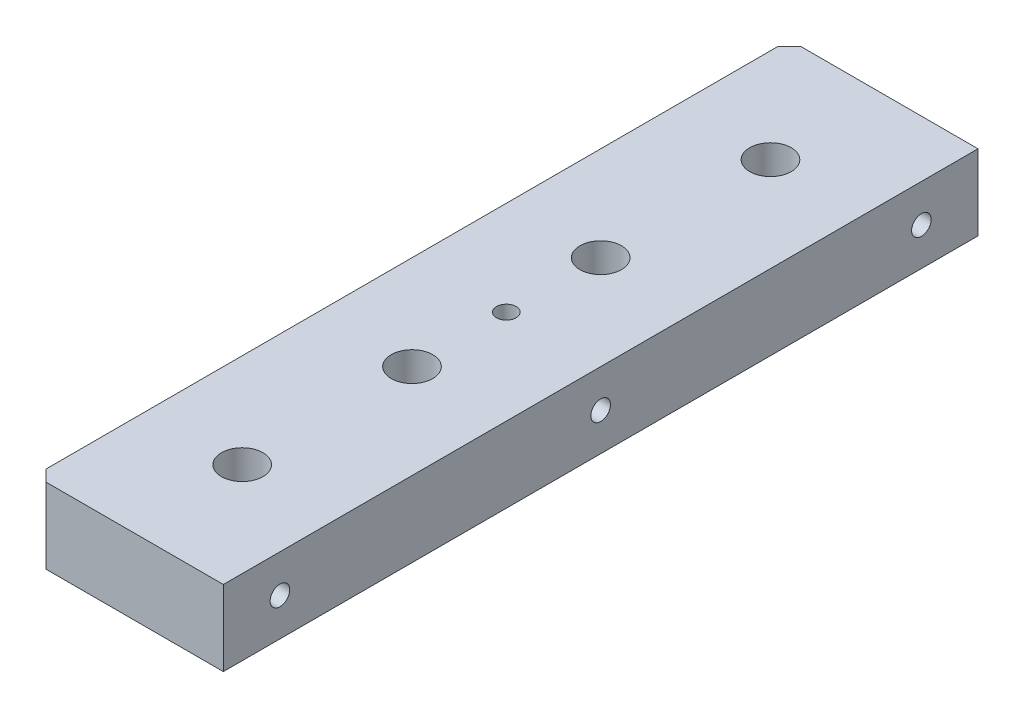
from build123d import *

# Parameters (mm, degrees)
SKETCH_1_W                   = 50
SKETCH_1_H                   = 200
EXTRUDE_1_DEPTH              = 10
HOLE_WIZARD_M6_1_D           = 6.6
HOLE_WIZARD_M6_1_CBORE_D     = 11
HOLE_WIZARD_M6_1_CBORE_DEPTH = 8
HOLE_WIZARD_M6_1_2_D         = 5.2
HOLE_WIZARD_M6_1_2_DEPTH     = 15
HOLE_WIZARD_M6_1_2_TIP       = 1.562237609
HOLE_WIZARD_M6_2_D           = 5.2
HOLE_WIZARD_M6_2_CBORE_D     = 11
HOLE_WIZARD_M6_2_CBORE_DEPTH = 6.4
CHAMFER_1_SIZE               = 3


with BuildPart() as part:
    # 草图1 → 凸台-拉伸1 (new, symmetric)
    with BuildSketch(Plane(origin=(0, 0, 0), x_dir=(1, 0, 0), z_dir=(0, 1, 0))):
        Rectangle(SKETCH_1_W, SKETCH_1_H)
    extrude(amount=EXTRUDE_1_DEPTH, both=True)

    # Hole Wizard M6 _1 (through all)
    with Locations(Plane(origin=(0, 10, 0), x_dir=(1, 0, 0), z_dir=(0, 1, 0))):
        with Locations((0, 70), (0, -70), (0, 25), (0, -25)):
            CounterBoreHole(HOLE_WIZARD_M6_1_D / 2, HOLE_WIZARD_M6_1_CBORE_D / 2, HOLE_WIZARD_M6_1_CBORE_DEPTH)

    # Hole Wizard M6 _1 2
    with Locations(Plane(origin=(25, 0, 0), x_dir=(0, 0, -1), z_dir=(1, 0, 0))):
        with Locations((-85, 0), (0, 0), (85, 0)):
            Hole(HOLE_WIZARD_M6_1_2_D / 2, depth=HOLE_WIZARD_M6_1_2_DEPTH)
            with Locations((0, 0, -(HOLE_WIZARD_M6_1_2_DEPTH + HOLE_WIZARD_M6_1_2_TIP / 2))):  # 118° drill point
                Cone(0, HOLE_WIZARD_M6_1_2_D / 2, HOLE_WIZARD_M6_1_2_TIP, mode=Mode.SUBTRACT)

    # M6 六角凹头螺钉的柱形沉头孔2 (through all)
    with Locations(Plane(origin=(0, -10, 0), x_dir=(-1, 0, 0), z_dir=(0, -1, 0))):
        with Locations((0, 0)):
            CounterBoreHole(HOLE_WIZARD_M6_2_D / 2, HOLE_WIZARD_M6_2_CBORE_D / 2, HOLE_WIZARD_M6_2_CBORE_DEPTH)

    # 倒角1
    chamfer_1_edges = [part.edges().sort_by_distance(p)[0] for p in [
        (-25, 0, -100),
        (-25, 0, 100),
    ]]
    chamfer(chamfer_1_edges, length=CHAMFER_1_SIZE)


solid = part.part
